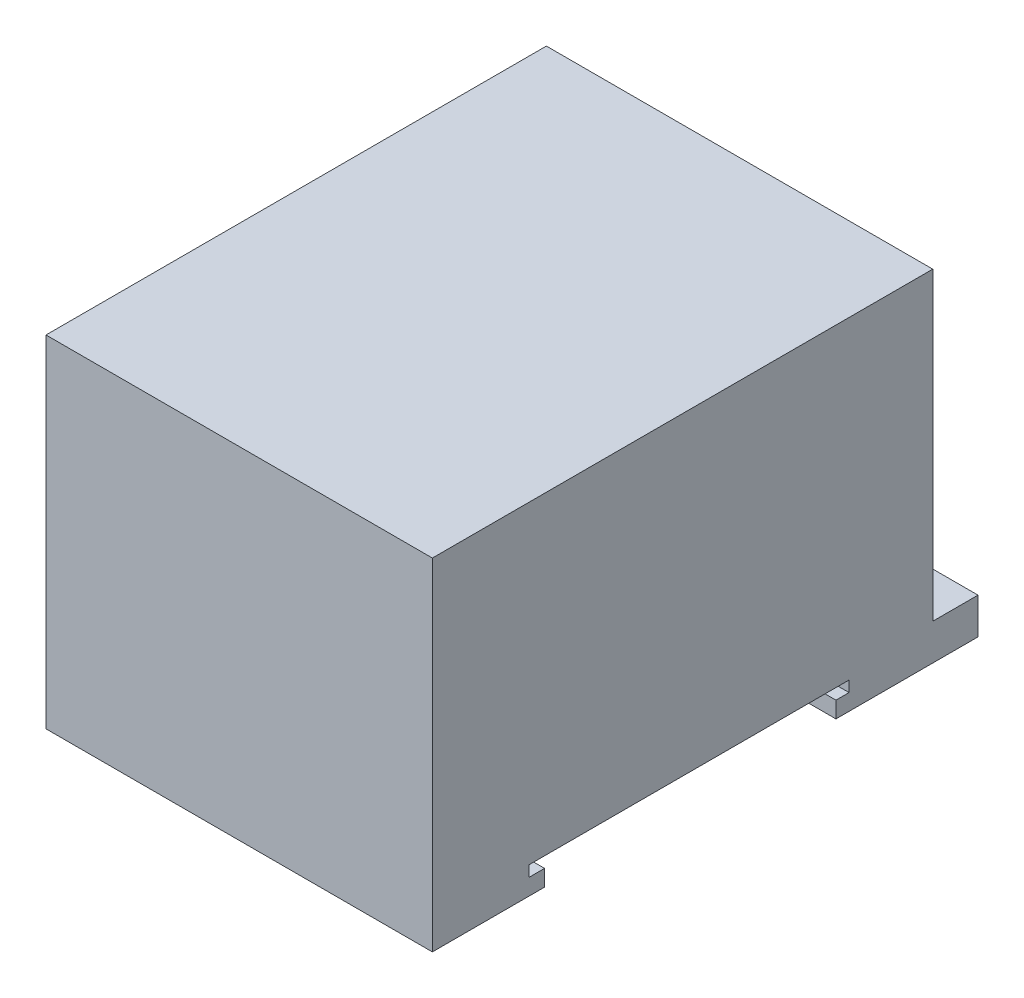
from build123d import *

# Parameters (mm, degrees)
SKETCH1_W           = 42.7
SKETCH1_H           = 55.3
BOSS_EXTRUDE1_DEPTH = 37.7
CUT_EXTRUDE1_REACH  = 65.317
SKETCH4_W           = 10
SKETCH4_H           = 5
BOSS_EXTRUDE2_DEPTH = 4


with BuildPart() as part:
    # Sketch1 → Boss-Extrude1 (new body)
    with BuildSketch(Plane(origin=(0, 0, 0), x_dir=(1, 0, 0), z_dir=(0, 1, 0))):
        Rectangle(SKETCH1_W, SKETCH1_H)
    extrude(amount=BOSS_EXTRUDE1_DEPTH)

    # Sketch3 → Cut-Extrude1 (cut, up to next)
    with BuildSketch(Plane(origin=(21.35, 0, 0), x_dir=(0, 0, -1), z_dir=(1, 0, 0)), mode=Mode.PRIVATE) as cut_extrude1_sk1:
        Polygon((-15.25, 0), (-15.25, 1.8), (-16.95, 1.8), (-16.95, 3), (18.399583247, 3), (18.399583247, 1.8), (16.95, 1.8), (16.95, 0), align=None)
    cut_extrude1_tool1 = extrude(cut_extrude1_sk1.sketch, amount=-CUT_EXTRUDE1_REACH, mode=Mode.PRIVATE) & part.part
    add(cut_extrude1_tool1.solids().sort_by_distance((21.35, 1.533887, -0.797088))[0], mode=Mode.SUBTRACT)

    # Sketch4 → Boss-Extrude2 (add)
    with BuildSketch(Plane.XZ):
        with Locations((16.35, -30.15)):
            Rectangle(SKETCH4_W, SKETCH4_H)
    extrude(amount=-BOSS_EXTRUDE2_DEPTH)


solid = part.part
